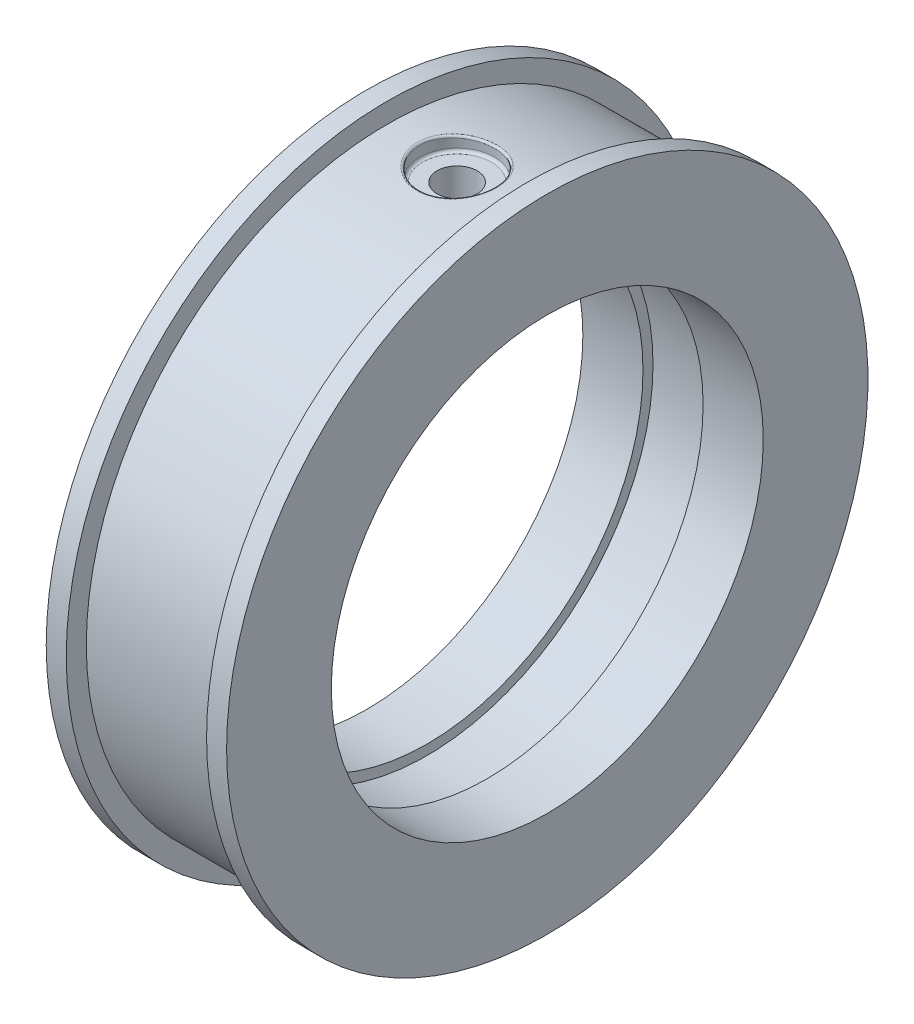
from build123d import *

# Parameters (mm, degrees)
HOLE1_D           = 7.5
HOLE1_DEPTH       = 1.5
HOLE2_REACH       = 71.113
HOLE2_BORE_R      = 2
DOWEL_HOLE1_D     = 4
DOWEL_HOLE1_DEPTH = 4
DOWEL_HOLE1_TIP   = 1.201721238
FILLET1_R         = 0.2
FILLET2_R         = 0.3


with BuildPart() as part:
    # Sketch1 → Revolve1 (revolve)
    with BuildSketch(Plane.XY, mode=Mode.PRIVATE) as revolve1_sk:
        Polygon((-8.389660143, 21.55), (-8.389660143, 32), (-6.389660143, 32), (-6.389660143, 30), (7.610339857, 30), (7.610339857, 32), (9.610339857, 32), (9.610339857, 21.55), (3.610339857, 21.55), (3.610339857, 22.55), (-2.389660143, 22.55), (-2.389660143, 21.55), align=None)
    revolve(revolve1_sk.sketch.rotate(Axis((-19.036826505, 0, 0), (1, 0, 0)), 90), axis=Axis((-19.036826505, 0, 0), (1, 0, 0)))

    # Hole1
    with Locations(Plane(origin=(0, 30, 0), x_dir=(1, 0, 0), z_dir=(0, 1, 0))):
        with Locations((0.610339857, 0)):
            Hole(HOLE1_D / 2, depth=HOLE1_DEPTH)

    # Hole2 bore → Hole2 (cut, up to next)
    with BuildSketch(Plane(origin=(0, 28.5, 0), x_dir=(1, 0, 0), z_dir=(0, 1, 0)), mode=Mode.PRIVATE) as hole2_sk1:
        with Locations((0.610339857, 0)):
            Circle(HOLE2_BORE_R)
    hole2_tool1 = extrude(hole2_sk1.sketch, amount=-HOLE2_REACH, mode=Mode.PRIVATE) & part.part
    add(hole2_tool1.solids().sort_by_distance((0.61034, 28.5, 0))[0], mode=Mode.SUBTRACT)

    # Dowel Hole1
    with Locations(Plane(origin=(0, -30, 0), x_dir=(-1, 0, 0), z_dir=(0, -1, 0))):
        with Locations((-0.610339857, 0)):
            Hole(DOWEL_HOLE1_D / 2, depth=DOWEL_HOLE1_DEPTH)
            with Locations((0, 0, -(DOWEL_HOLE1_DEPTH + DOWEL_HOLE1_TIP / 2))):  # 118° drill point
                Cone(0, DOWEL_HOLE1_D / 2, DOWEL_HOLE1_TIP, mode=Mode.SUBTRACT)

    # Fillet1
    fillet1_edges = [part.edges().sort_by_distance(p)[0] for p in [
        (4.360339864, 29.999999997, -1e-09),
    ]]
    fillet(fillet1_edges, radius=FILLET1_R)

    # Fillet2
    fillet2_edges = [part.edges().sort_by_distance(p)[0] for p in [
        (4.360339857, 28.5, 0),
    ]]
    fillet(fillet2_edges, radius=FILLET2_R)


solid = part.part
